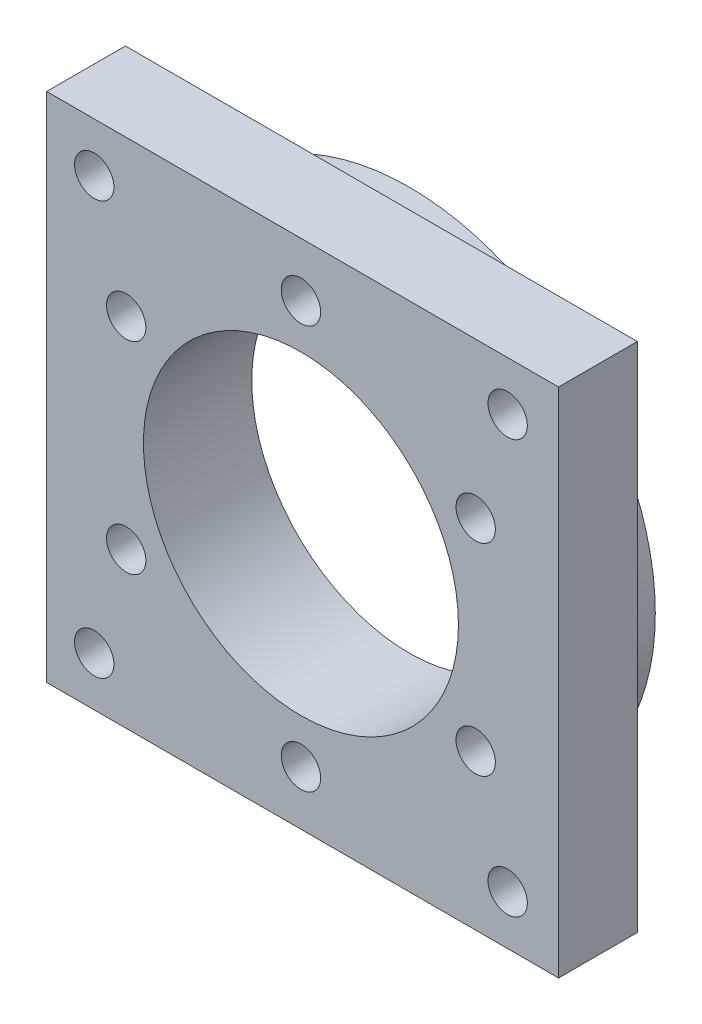
SolidWorks part; units mm, degrees
ref_plane "Front Plane" through (0, 0, 0) normal (0, 0, 1) x (1, 0, 0)
ref_plane "Top Plane" through (0, 0, 0) normal (0, 1, 0) x (1, 0, 0)
ref_plane "Right Plane" through (0, 0, 0) normal (1, 0, 0) x (0, 0, -1)
other "Configuration Table"
sketch "Sketch1" plane through (0, 0, 0) normal (0, 0, 1) x (1, 0, 0)
  circle A0 centre (0, 0) radius 16
  circle A1 centre (0, 0) radius 25
  dimension "D1" = 32
  dimension "D2" = 50
extrude "Boss-Extrude1" add sketch "Sketch1" along normal blind 3
sketch "Sketch2" plane through (0, 0, 3) normal (0, 0, 1) x (1, 0, 0)
  line L0 (-47.2299, 0) -> (45.2747, 0) construction
  line L1 (-25.8296, 26) -> (26.1704, 26)
  line L2 (-25.8296, 26) -> (-25.8296, -26)
  line L3 (-25.8296, -26) -> (26.1704, -26)
  line L4 (26.1704, 26) -> (26.1704, -26)
  line L5 (0, 42.3444) -> (0, -42.6225) construction
  circle A0 centre (0, 0) radius 16
  dimension "D1" = 52
  dimension "D2" = 52
extrude "Boss-Extrude2" add sketch "Sketch2" along normal blind 8
sketch "Sketch3" plane through (0, 0, 0) normal (0, 0, -1) x (-1, 0, 0)
  circle A0 centre (0, 0) radius 20.5 construction
  circle A1 centre (0, 20.5) radius 2
  circle A2 centre (17.7535, 10.25) radius 2
  circle A3 centre (17.7535, -10.25) radius 2
  circle A4 centre (0, -20.5) radius 2
  circle A5 centre (-17.7535, -10.25) radius 2
  circle A6 centre (-17.7535, 10.25) radius 2
  point P18 (0, 0)
  dimension "D1" = 41
  dimension "D2" = 4
  dimension "D3" = 6
extrude "Cut-Extrude1" cut sketch "Sketch3" against normal through all
sketch "Sketch4" plane through (0, 0, 3) normal (0, 0, -1) x (-1, 0, 0)
  line L0 (-36.1924, 0) -> (0, 0) construction
  line L1 (0, 0) -> (0, 38.9189) construction
  circle A0 centre (-21, 21) radius 2
  circle A4 centre (21, 21) radius 2
  circle A5 centre (21, -21) radius 2
  circle A6 centre (-21, -21) radius 2
  dimension "D1" = 4
  dimension "D2" = 21
  dimension "D3" = 21
extrude "Cut-Extrude2" cut sketch "Sketch4" against normal through all
sketch "Sketch5" plane through (0, 0, 0) normal (0, 0, -1) x (-1, 0, 0)
  circle A0 centre (0, 20.5) radius 3.5
  circle A1 centre (17.7535, 10.25) radius 3.5
  circle A2 centre (17.7535, -10.25) radius 3.5
  circle A3 centre (0, -20.5) radius 3.5
  circle A4 centre (-17.7535, -10.25) radius 3.5
  circle A5 centre (-17.7535, 10.25) radius 3.5
  point P15 (0, 0)
  dimension "D1" = 7
  dimension "D2" = 6
extrude "Cut-Extrude3" cut sketch "Sketch5" against normal blind 3
